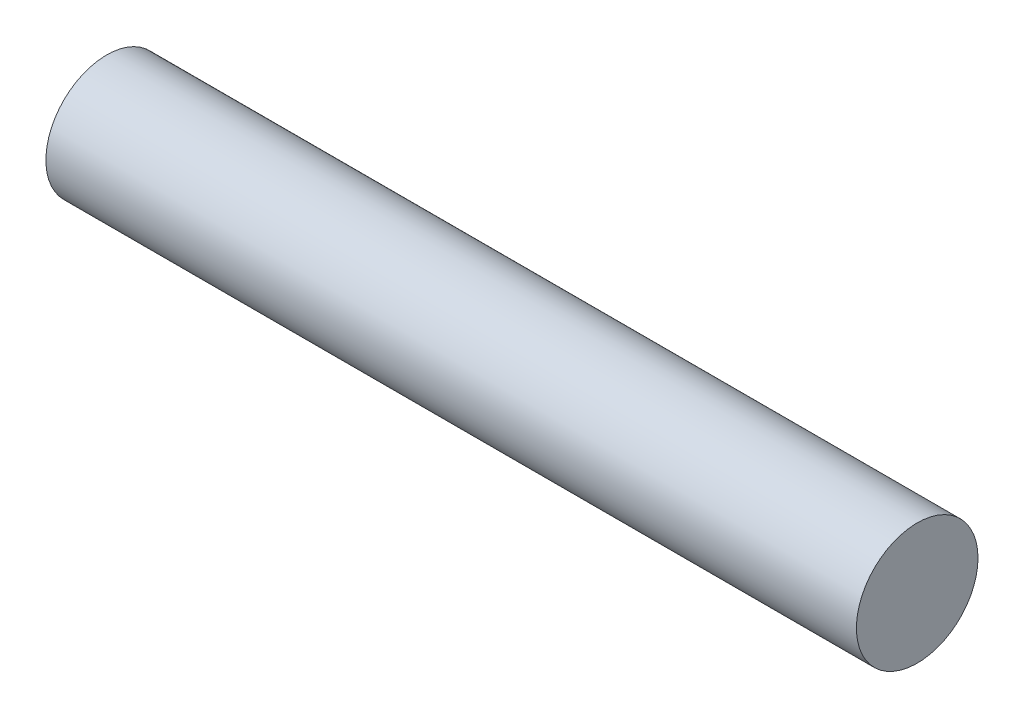
from build123d import *

# Parameters (mm, degrees)
SKETCH1_R           = 1.5
BOSS_EXTRUDE1_DEPTH = 20


with BuildPart() as part:
    # Sketch1 → Boss-Extrude1 (new body)
    with BuildSketch(Plane(origin=(0, 0, 0), x_dir=(0, 0, -1), z_dir=(1, 0, 0))):
        Circle(SKETCH1_R)
    extrude(amount=BOSS_EXTRUDE1_DEPTH)


solid = part.part
